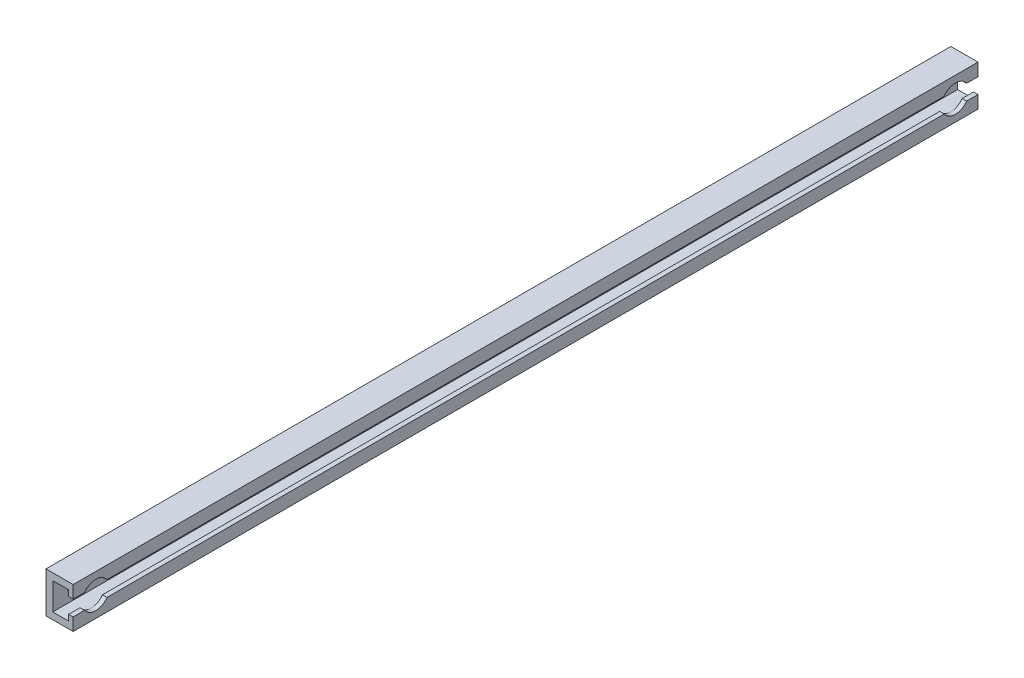
from build123d import *

# Parameters (mm, degrees)
EXTRUDE_1_DEPTH     = 200
CUT_EXTRUDE_1_DEPTH = 0.1
SKETCH_3_R          = 3
CUT_EXTRUDE_2_DEPTH = 4.5
SKETCH_4_R          = 1.75
CUT_EXTRUDE_3_DEPTH = 261.9000942


with BuildPart() as part:
    # Model → 凸台-拉伸1 (new body)
    with BuildSketch(Plane.XY):
        Polygon((235.971352115, 159.97718973), (239.471352115, 159.97718973), (239.471352115, 161.27718973), (240.471352115, 161.27718973), (240.471352115, 158.47718973), (234.471352115, 158.47718973), (234.471352115, 167.47718973), (240.471352115, 167.47718973), (240.471352115, 164.67718973), (239.471352115, 164.67718973), (239.471352115, 165.97718973), (235.971352115, 165.97718973), align=None)
    extrude(amount=EXTRUDE_1_DEPTH)

    # 草图2 → 切除-拉伸1 (cut)
    with BuildSketch(Plane(origin=(234.471352115, 157.934205003, -3.551128869), x_dir=(0, 0, 1), z_dir=(-1, 0, 0))):
        with BuildLine():
            Line((12.414790076, 6.667469393), (12.914790076, 6.667469393))
            add(Edge.make_bspline(
                [(12.914790076, 6.667469393), (13.105445322, 8.024946973), (11.817726071, 7.304400271), (10.53000682, 6.583853569), (11.375222173, 5.806000114), (12.220437527, 5.02814666), (12.828246359, 6.37441634)],
                knots=[2.310776883, 2.310776883, 2.310776883, 4.295504112, 4.295504112, 6.280231341, 6.280231341, 8.26495857, 8.26495857, 8.26495857], degree=2, weights=[1, 0.546712287, 1, 0.546712287, 1, 0.546712287, 1]))
            Line((12.828246359, 6.37441634), (12.235749287, 6.37441634))
            add(Edge.make_bspline(
                [(12.414790076, 6.667469393), (12.579589729, 7.17892596), (12.071440891, 6.880567221), (11.563292052, 6.582208482), (11.676360556, 6.233901737), (11.789429059, 5.885594992), (12.235749287, 6.37441634)],
                knots=[2.310776883, 2.310776883, 2.310776883, 4.1585118, 4.1585118, 6.006246717, 6.006246717, 7.853981634, 7.853981634, 7.853981634], degree=2, weights=[1, 0.602738677, 1, 0.602738677, 1, 0.602738677, 1]))
        make_face()
        Polygon((10.199062367, 6.100160833), (10.830142798, 7.438022654), (10.330142798, 7.438022654), (9.485749287, 5.647946802), (10.735749287, 5.647946802), (10.949062367, 6.100160833), align=None)
        Polygon((8.82776943, 6.587639422), (8.485749287, 5.647946802), (7.985749287, 5.647946802), (8.32776943, 6.587639422), (7.985749287, 7.438022654), (8.485749287, 7.438022654), (8.690961373, 6.927792715), (9.235749287, 7.438022654), (9.735749287, 7.438022654), align=None)
        with BuildLine():
            add(Edge.make_bspline(
                [(7.246674356, 7.580632375), (6.380164872, 8.195748474), (5.694823482, 7.059454556)],
                knots=[6.223464168, 6.223464168, 6.223464168, 7.853981634, 7.853981634, 7.853981634], degree=2, weights=[1, 0.685680084, 1]))
            add(Edge.make_bspline(
                [(7.740648551, 7.658024201), (7.149045607, 9.470550368), (5.694823482, 7.059454556)],
                knots=[5.824568949, 5.824568949, 5.824568949, 7.853981634, 7.853981634, 7.853981634], degree=2, weights=[1, 0.527869365, 1]))
            Line((7.740648551, 7.658024201), (7.246674356, 7.580632375))
        make_face()
        with BuildLine():
            Line((6.924255788, 6.700667335), (7.422353137, 6.744245207))
            add(Edge.make_bspline(
                [(7.422353137, 6.744245207), (7.566792843, 9.328849149), (5.887544801, 6.911260491), (4.208296758, 4.493671833), (6.735749287, 5.755751762)],
                knots=[5.539635999, 5.539635999, 5.539635999, 8.030367113, 8.030367113, 10.521098226, 10.521098226, 10.521098226], degree=2, weights=[1, 0.319716976, 1, 0.319716976, 1]))
            Line((6.735749287, 5.755751762), (6.735749287, 5.647946802))
            Line((6.735749287, 5.647946802), (6.985749287, 5.647946802))
            Line((6.985749287, 5.647946802), (7.42055637, 6.569718047))
            Line((7.42055637, 6.569718047), (6.575537831, 6.569718047))
            Line((6.575537831, 6.569718047), (6.460496551, 6.347759709))
            Line((6.460496551, 6.347759709), (6.710496551, 6.347759709))
            add(Edge.make_bspline(
                [(6.924255788, 6.700667335), (7.039891919, 7.169169172), (6.558503894, 6.872786595), (6.07711587, 6.576404017), (6.174734812, 6.239199772), (6.272353754, 5.901995526), (6.710496551, 6.347759709)],
                knots=[5.539635999, 5.539635999, 5.539635999, 7.333784926, 7.333784926, 9.127933854, 9.127933854, 10.922082781, 10.922082781, 10.922082781], degree=2, weights=[1, 0.623898956, 1, 0.623898956, 1, 0.623898956, 1]))
        make_face()
        with BuildLine():
            add(Edge.make_bspline(
                [(5.855583383, 5.505337081), (6.722092867, 4.890220982), (7.407434257, 6.0265149)],
                knots=[3.081871514, 3.081871514, 3.081871514, 4.71238898, 4.71238898, 4.71238898], degree=2, weights=[1, 0.685680084, 1]))
            add(Edge.make_bspline(
                [(5.361609188, 5.427945255), (5.953212132, 3.615419087), (7.407434257, 6.0265149)],
                knots=[2.682976295, 2.682976295, 2.682976295, 4.71238898, 4.71238898, 4.71238898], degree=2, weights=[1, 0.527869365, 1]))
            Line((5.361609188, 5.427945255), (5.855583383, 5.505337081))
        make_face()
    extrude(amount=-CUT_EXTRUDE_1_DEPTH, mode=Mode.SUBTRACT)

    # 草图3 → 切除-拉伸2 (cut)
    with BuildSketch(Plane(origin=(240.471352115, 0, 0), x_dir=(0, 0, -1), z_dir=(1, 0, 0))):
        with Locations((-195, 162.97718973)):
            Circle(SKETCH_3_R)
        with Locations((-5, 162.97718973)):
            Circle(SKETCH_3_R)
    extrude(amount=-CUT_EXTRUDE_2_DEPTH, mode=Mode.SUBTRACT)

    # 草图4 → 切除-拉伸3 (cut, through all)
    with BuildSketch(Plane(origin=(235.971352115, 0, 0), x_dir=(0, 0, -1), z_dir=(1, 0, 0))):
        with Locations((-195, 162.97718973)):
            Circle(SKETCH_4_R)
        with Locations((-5, 162.97718973)):
            Circle(SKETCH_4_R)
    extrude(amount=-CUT_EXTRUDE_3_DEPTH, mode=Mode.SUBTRACT)


solid = part.part
